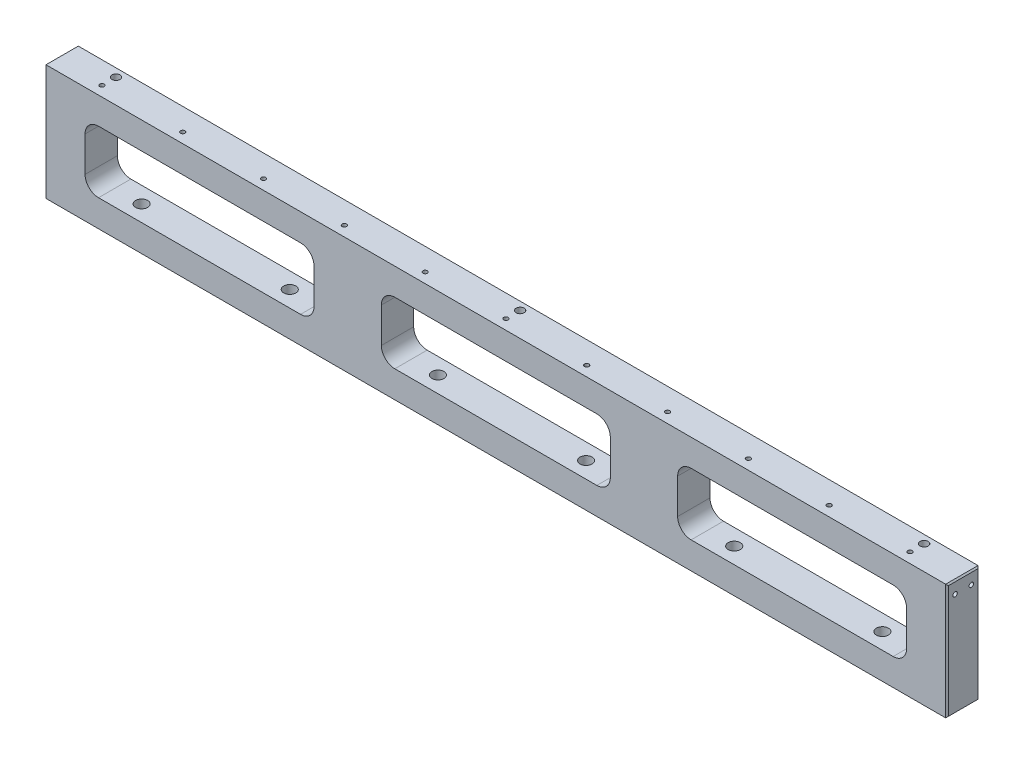
SolidWorks part; units mm, degrees
material "AL6061"
ref_plane "Front" through (0, 0, 0) normal (0, 0, 1) x (1, 0, 0)
ref_plane "Top" through (0, 0, 0) normal (0, 1, 0) x (1, 0, 0)
ref_plane "Right" through (0, 0, 0) normal (1, 0, 0) x (0, 0, -1)
sketch "Sketch1" plane through (0, 0, 0) normal (0, 0, 1) x (1, 0, 0)
  line L1 (-335, -43) -> (335, -43)
  line L2 (-335, -43) -> (-335, 43)
  line L3 (-335, 43) -> (335, 43)
  line L4 (335, -43) -> (335, 43)
  line L5 (-335, -43) -> (335, 43) construction
  line L6 (-335, 43) -> (335, -43) construction
  point P0 (0, 0)
  dimension "D1" = 670
  dimension "D2" = 86
extrude "Boss-Extrude1" add sketch "Sketch1" along normal mid plane 24
sketch "Sketch2" plane through (0, 0, 12) normal (0, 0, 1) x (1, 0, 0)
  line L0 (-335, -43) -> (335, -43) construction
  line L1 (-295, 23) -> (-145, 23)
  line L2 (-305, 13) -> (-305, -13)
  line L3 (-295, -23) -> (-145, -23)
  line L4 (-135, 13) -> (-135, -13)
  line L5 (-335, 43) -> (-335, -43) construction
  line L6 (-75, 23) -> (75, 23)
  line L7 (-85, 13) -> (-85, -13)
  line L8 (-75, -23) -> (75, -23)
  line L9 (85, 13) -> (85, -13)
  line L10 (145, 23) -> (295, 23)
  line L11 (135, 13) -> (135, -13)
  line L12 (145, -23) -> (295, -23)
  line L13 (305, 13) -> (305, -13)
  line L14 (-295, 23) -> (-75, 23) construction
  line L15 (335, -43) -> (335, 43) construction
  line L16 (335, 43) -> (-335, 43) construction
  arc A0 (-305, -13) -> (-295, -23) centre (-295, -13) ccw
  arc A1 (-145, -23) -> (-135, -13) centre (-145, -13) ccw
  arc A2 (-135, 13) -> (-145, 23) centre (-145, 13) ccw
  arc A3 (-295, 23) -> (-305, 13) centre (-295, 13) ccw
  arc A4 (-85, -13) -> (-75, -23) centre (-75, -13) ccw
  arc A5 (75, -23) -> (85, -13) centre (75, -13) ccw
  arc A6 (85, 13) -> (75, 23) centre (75, 13) ccw
  arc A7 (-75, 23) -> (-85, 13) centre (-75, 13) ccw
  arc A8 (135, -13) -> (145, -23) centre (145, -13) ccw
  arc A9 (295, -23) -> (305, -13) centre (295, -13) ccw
  arc A10 (305, 13) -> (295, 23) centre (295, 13) ccw
  arc A11 (145, 23) -> (135, 13) centre (145, 13) ccw
  point P10 (-305, -23)
  point P13 (-135, -23)
  dimension "D5" = 10
  dimension "D1" = 170
  dimension "D2" = 20
  dimension "D3" = 20
  dimension "D4" = 30
  dimension "D7" = 220
  dimension "D8" = 30
  dimension "D6" = 3
extrude "Cut-Extrude1" cut sketch "Sketch2" against normal through all
hole_wizard "M8 Clearance Hole1" positions "Sketch3" profile "Sketch4" hole size "M8" standard "GB"
sketch "Sketch3" plane through (0, -43, 0) normal (0, -1, 0) x (-1, 0, 0)
  line L0 (0, 0) -> (304.414, 0) construction
  line L3 (220, 0) -> (220, -52.9643) construction
  line L6 (305, 12) -> (305, -12) construction
  line L7 (135, 12) -> (135, -12) construction
  line L8 (165, 0) -> (-55, 0) construction
  point P15 (275, 0)
  point P18 (165, 0)
  point P23 (55, 0)
  point P24 (-55, 0)
  point P25 (-165, 0)
  point P26 (-275, 0)
  dimension "D1" = 110
  dimension "D3" = 220
  dimension "D2" = 3
sketch "Sketch4" plane through (275, -43, 0) normal (1, 0, 0) x (0, 0, -1)
  line L0 (0, 0) -> (0, 20)
  line L1 (0, 20) -> (4.5, 20)
  line L2 (4.5, 20) -> (4.5, 0)
  line L5 (4.5, 0) -> (0, 0)
  line L11 (0, -6.35) -> (0, 107.95) construction
  dimension "通孔孔直径" = 9
  dimension "通孔孔深度" = 20
hole_wizard "M4 Tapped Hole1" positions "Sketch5" profile "Sketch6" tap size "M4" standard "GB"
sketch "Sketch5" plane through (0, 43, 0) normal (0, 1, 0) x (1, 0, 0)
  line L0 (-335, -12) -> (-335, 12) construction
  line L1 (335, -12) -> (-335, -12) construction
  line L2 (-300, -4.5) -> (-240, -4.5) construction
  point P0 (-300, -4.5)
  point P11 (-240, -4.5)
  point P12 (-180, -4.5)
  point P13 (-120, -4.5)
  point P14 (-60, -4.5)
  point P15 (0, -4.5)
  point P16 (60, -4.5)
  point P17 (120, -4.5)
  point P18 (180, -4.5)
  point P19 (240, -4.5)
  point P22 (300, -4.5)
  dimension "D1" = 35
  dimension "D2" = 7.5
  dimension "D4" = 60
  dimension "D3" = 11
sketch "Sketch6" plane through (-300, 43, 4.5) normal (1, 0, 0) x (0, 0, 1)
  line L0 (0, 0) -> (0, 11.0914)
  line L1 (0, 11.0914) -> (1.65, 10.1)
  line L2 (1.65, 10.1) -> (1.65, 0)
  line L5 (1.65, 0) -> (0, 0)
  line L10 (0, 11.0914) -> (-1.65, 10.1) construction
  line L11 (0, -6.35) -> (0, 107.95) construction
  dimension "螺纹孔钻头直径" = 3.3
  dimension "螺纹孔钻头深度" = 10.1
  dimension "导头角度" = 118
cosmetic thread "Cosmetic Thread7" parameters "D1"=8, "D2"=4
cosmetic thread "Cosmetic Thread8" parameters "D1"=8, "D2"=4
cosmetic thread "Cosmetic Thread9" parameters "D1"=8, "D2"=4
cosmetic thread "Cosmetic Thread10" parameters "D1"=8, "D2"=4
cosmetic thread "Cosmetic Thread11" parameters "D1"=8, "D2"=4
cosmetic thread "Cosmetic Thread12" parameters "D1"=8, "D2"=4
cosmetic thread "Cosmetic Thread13" parameters "D1"=8, "D2"=4
cosmetic thread "Cosmetic Thread14" parameters "D1"=8, "D2"=4
cosmetic thread "Cosmetic Thread15" parameters "D1"=8, "D2"=4
cosmetic thread "Cosmetic Thread16" parameters "D1"=8, "D2"=4
cosmetic thread "Cosmetic Thread21" parameters "D1"=8, "D2"=4
hole_wizard "Dowel Hole1" positions "Sketch7" profile "Sketch8" hole size "Ø6.0" standard "GB"
sketch "Sketch7" plane through (0, 43, 0) normal (0, 1, 0) x (1, 0, 0)
  line L0 (-300, -4.5) -> (-300, 14.7507) construction
  line L1 (-300, 6) -> (0, 6) construction
  circle A0 centre (-300, -4.5) radius 1.65 construction
  point P8 (-300, 6)
  point P17 (0, 6)
  point P18 (300, 6)
  dimension "D1" = 10.5
  dimension "D3" = 300
  dimension "D2" = 3
sketch "Sketch8" plane through (300, 43, -6) normal (1, 0, 0) x (0, 0, 1)
  line L0 (0, 0) -> (0, 11.9026)
  line L1 (0, 11.9026) -> (3, 10.1)
  line L2 (3, 10.1) -> (3, 0)
  line L5 (3, 0) -> (0, 0)
  line L10 (0, 11.9026) -> (-3, 10.1) construction
  line L11 (0, -6.35) -> (0, 107.95) construction
  dimension "孔直径" = 6
  dimension "孔深度" = 10.1
  dimension "导头角度" = 118
chamfer "Chamfer1" distance 1 angle 45 8 edges at (-335, 43, 0) (-335, 0, 12) (-335, -43, 0) (-335, 0, -12) (335, -43, 0) (335, 0, 12) (335, 43, 0) (335, 0, -12)
hole_wizard "M4 Tapped Hole2" positions "Sketch9" profile "Sketch10" tap size "M4" standard "GB"
sketch "Sketch9" plane through (-335, 0, 0) normal (-1, 0, 0) x (0, 0, 1)
  line L0 (0, 0) -> (0, 57.5879) construction
  line L1 (-12, 43) -> (12, 43) construction
  point P7 (-6, 34)
  point P10 (6, 34)
  dimension "D1" = 12
  dimension "D2" = 9
sketch "Sketch10" plane through (-335, 34, 6) normal (0, 1, 0) x (0, 0, 1)
  line L0 (0, 0) -> (0, 11.0914)
  line L1 (0, 11.0914) -> (1.65, 10.1)
  line L2 (1.65, 10.1) -> (1.65, 0)
  line L5 (1.65, 0) -> (0, 0)
  line L10 (0, 11.0914) -> (-1.65, 10.1) construction
  line L11 (0, -6.35) -> (0, 107.95) construction
  dimension "螺纹孔钻头直径" = 3.3
  dimension "螺纹孔钻头深度" = 10.1
  dimension "导头角度" = 118
cosmetic thread "Cosmetic Thread17" parameters "D1"=8, "D2"=4
cosmetic thread "Cosmetic Thread18" parameters "D1"=8, "D2"=4
hole_wizard "M4 Tapped Hole3" positions "Sketch11" profile "Sketch12" tap size "M4" standard "GB"
sketch "Sketch11" plane through (335, 0, 0) normal (1, 0, 0) x (0, 0, -1)
  point P0 (-6, 34)
  point P3 (6, 34)
sketch "Sketch12" plane through (335, 34, 6) normal (0, 1, 0) x (0, 0, -1)
  line L0 (0, 0) -> (0, 11.0914)
  line L1 (0, 11.0914) -> (1.65, 10.1)
  line L2 (1.65, 10.1) -> (1.65, 0)
  line L5 (1.65, 0) -> (0, 0)
  line L10 (0, 11.0914) -> (-1.65, 10.1) construction
  line L11 (0, -6.35) -> (0, 107.95) construction
  dimension "螺纹孔钻头直径" = 3.3
  dimension "螺纹孔钻头深度" = 10.1
  dimension "导头角度" = 118
cosmetic thread "Cosmetic Thread19" parameters "D1"=8, "D2"=4
cosmetic thread "Cosmetic Thread20" parameters "D1"=8, "D2"=4
